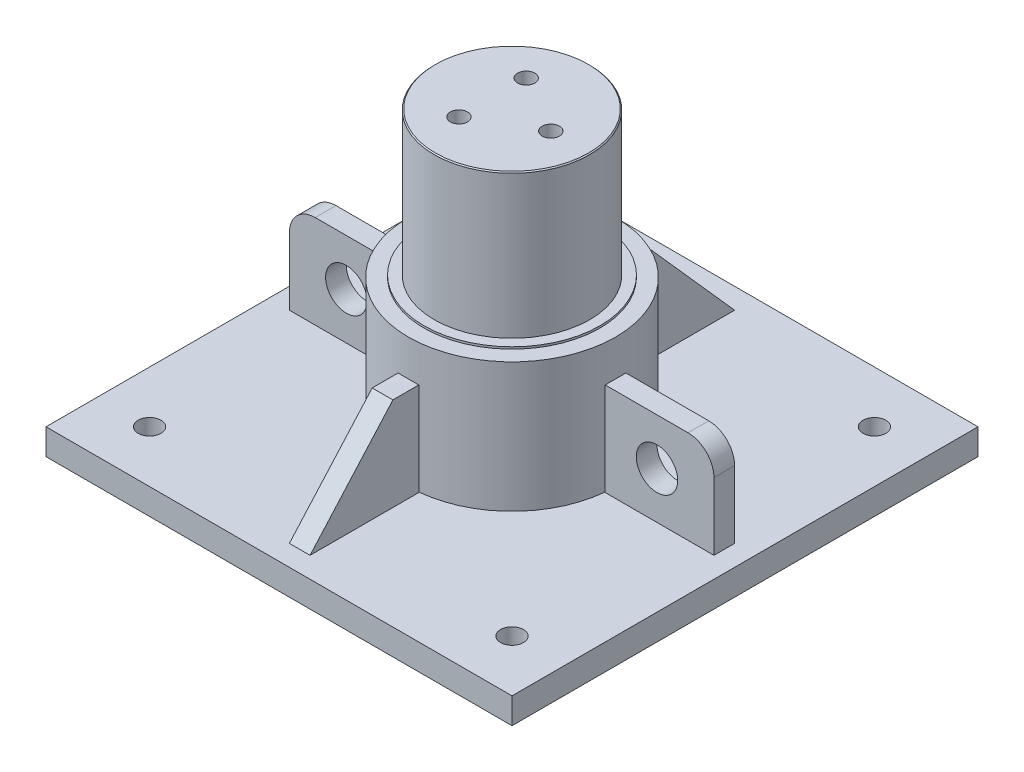
from build123d import *

# Parameters (mm, degrees)
SKETCH1_W               = 450
SKETCH1_H               = 450
SKETCH1_R               = 100
BOSS_EXTRUDE1_DEPTH     = 25
SKETCH2_R               = 100
BOSS_EXTRUDE2_DEPTH     = 150
SKETCH3_R               = 85
BOSS_EXTRUDE3_DEPTH     = 2
SKETCH4_R               = 75
BOSS_EXTRUDE4_DEPTH     = 139
SKETCH5_R               = 11
CUT_EXTRUDE1_DEPTH      = 415.736060646
CIRPATTERN1_COUNT       = 3
CHAMFER1_SIZE           = 1
SKETCH8_W               = 105
SKETCH8_H               = 90
BOSS_EXTRUDE5_DEPTH     = 10
BOSS_EXTRUDE5_2_DEPTH   = 10
FILLET1_R               = 25
FILLET2_R               = 25
CUT_EXTRUDE2_DEPTH      = 437.498568153
CUT_EXTRUDE2_DEPTH_BACK = 437.498568153
SKETCH9_R               = 20
BOSS_EXTRUDE6_DEPTH     = 10
BOSS_EXTRUDE6_2_DEPTH   = 10


with BuildPart() as part:
    # Sketch1 → Boss-Extrude1 (new body)
    with BuildSketch(Plane(origin=(0, 0, 0), x_dir=(1, 0, 0), z_dir=(0, 1, 0))):
        Rectangle(SKETCH1_W, SKETCH1_H)
        with Locations(Location((0, 0, 0), (0, 0, 270))):
            Circle(SKETCH1_R, mode=Mode.SUBTRACT)
    extrude(amount=BOSS_EXTRUDE1_DEPTH)

    # Sketch5 → Cut-Extrude1 (cut, through all)
    with BuildSketch(Plane(origin=(0, 25, 0), x_dir=(1, 0, 0), z_dir=(0, 1, 0))):
        with Locations(Location((-175, 175, 0), (0, 0, 270))):
            Circle(SKETCH5_R)
        with Locations(Location((175, 175, 0), (0, 0, 270))):
            Circle(SKETCH5_R)
        with Locations(Location((175, -175, 0), (0, 0, 270))):
            Circle(SKETCH5_R)
        with Locations(Location((-175, -175, 0), (0, 0, 270))):
            Circle(SKETCH5_R)
    extrude(amount=-CUT_EXTRUDE1_DEPTH, mode=Mode.SUBTRACT)


with BuildPart() as body_2:
    # Sketch2 → Boss-Extrude2 (new body)
    with BuildSketch(Plane.XZ):
        with Locations(Location((0, 0, 0), (0, 0, 270))):
            Circle(SKETCH2_R)
    extrude(amount=-BOSS_EXTRUDE2_DEPTH)

    # Sketch3 → Boss-Extrude3 (add)
    with BuildSketch(Plane(origin=(0, 150, 0), x_dir=(1, 0, 0), z_dir=(0, 1, 0))):
        with Locations(Location((0, 0, 0), (0, 0, 90))):
            Circle(SKETCH3_R)
    extrude(amount=BOSS_EXTRUDE3_DEPTH)

    # Sketch4 → Boss-Extrude4 (add)
    with BuildSketch(Plane(origin=(0, 152, 0), x_dir=(1, 0, 0), z_dir=(0, 1, 0))):
        with Locations(Location((0, 0, 0), (0, 0, 270))):
            Circle(SKETCH4_R)
    extrude(amount=BOSS_EXTRUDE4_DEPTH)

    # Sketch7 → 3/4-10 Tapped Hole1 (revolve, cut)
    with BuildSketch(Plane(origin=(37.5, 291, 0), x_dir=(0, 0, 1), z_dir=(1, 0, 0))):
        Polygon((0, 0), (0, 35.007416175), (8.33374, 30), (8.33374, 0), align=None)
    f_3_4_10_tapped_hole1 = revolve(axis=Axis((37.5, 297.35, 0), (0, -1, 0)), mode=Mode.SUBTRACT)

    # CirPattern1: 3/4-10 Tapped Hole1 ×3 about axis
    cirpattern1_axis = Axis((0, 0, 0), (0, 1, 0))
    for i in range(1, CIRPATTERN1_COUNT):
        add(f_3_4_10_tapped_hole1.rotate(cirpattern1_axis, i * 360 / CIRPATTERN1_COUNT), mode=Mode.SUBTRACT)

    # Chamfer1
    chamfer1_edges = [body_2.edges().sort_by_distance(p)[0] for p in [
        (0, 291, -75),
    ]]
    chamfer(chamfer1_edges, length=CHAMFER1_SIZE)


with BuildPart() as body_3:
    # Sketch8 → Boss-Extrude5 (new, symmetric)
    with BuildSketch(Plane.XY):
        with Locations((-152.5, 70)):
            Rectangle(SKETCH8_W, SKETCH8_H)
    extrude(amount=BOSS_EXTRUDE5_DEPTH, both=True)

    # Fillet1
    fillet1_edges = [body_3.edges().sort_by_distance(p)[0] for p in [
        (-205, 115, 0),
    ]]
    fillet(fillet1_edges, radius=FILLET1_R)


with BuildPart() as body_4:
    # Sketch8 → Boss-Extrude5 2 (new, symmetric)
    with BuildSketch(Plane.XY):
        with Locations((152.5, 70)):
            Rectangle(SKETCH8_W, SKETCH8_H)
    extrude(amount=BOSS_EXTRUDE5_2_DEPTH, both=True)

    # Fillet2
    fillet2_edges = [body_4.edges().sort_by_distance(p)[0] for p in [
        (205, 115, 0),
    ]]
    fillet(fillet2_edges, radius=FILLET2_R)


with BuildPart() as cut_extrude2_tool:
    # Sketch9 → Cut-Extrude2 (new, two sides: drawn at the far end of the back side and taken through both)
    with BuildSketch(Plane.XY.offset(10).offset(-CUT_EXTRUDE2_DEPTH_BACK)):
        with Locations(Location((-150, 70, 0), (0, 0, 180))):
            Circle(SKETCH9_R)
        with Locations((150, 70)):
            Circle(SKETCH9_R)
    extrude(amount=CUT_EXTRUDE2_DEPTH + CUT_EXTRUDE2_DEPTH_BACK)


with BuildPart() as body_3_1:
    add(body_3.part)

    # Cut-Extrude2: cut by cut_extrude2_tool
    add(cut_extrude2_tool.part, mode=Mode.SUBTRACT)


with BuildPart() as body_4_1:
    add(body_4.part)

    # Cut-Extrude2: cut by cut_extrude2_tool
    add(cut_extrude2_tool.part, mode=Mode.SUBTRACT)


with BuildPart() as body_5:
    # Sketch10 → Boss-Extrude6 (new, symmetric)
    with BuildSketch(Plane(origin=(0, 0, 0), x_dir=(0, 0, -1), z_dir=(1, 0, 0))):
        Polygon((-100, 25), (-205, 25), (-125, 115), (-100, 115), align=None)
    extrude(amount=BOSS_EXTRUDE6_DEPTH, both=True)


with BuildPart() as body_6:
    # Sketch10 → Boss-Extrude6 2 (new, symmetric)
    with BuildSketch(Plane(origin=(0, 0, 0), x_dir=(0, 0, -1), z_dir=(1, 0, 0))):
        Polygon((100, 115), (100, 25), (205, 25), (125, 115), align=None)
    extrude(amount=BOSS_EXTRUDE6_2_DEPTH, both=True)


solid = Compound([part.part, body_2.part, body_3_1.part, body_4_1.part, body_5.part, body_6.part])
